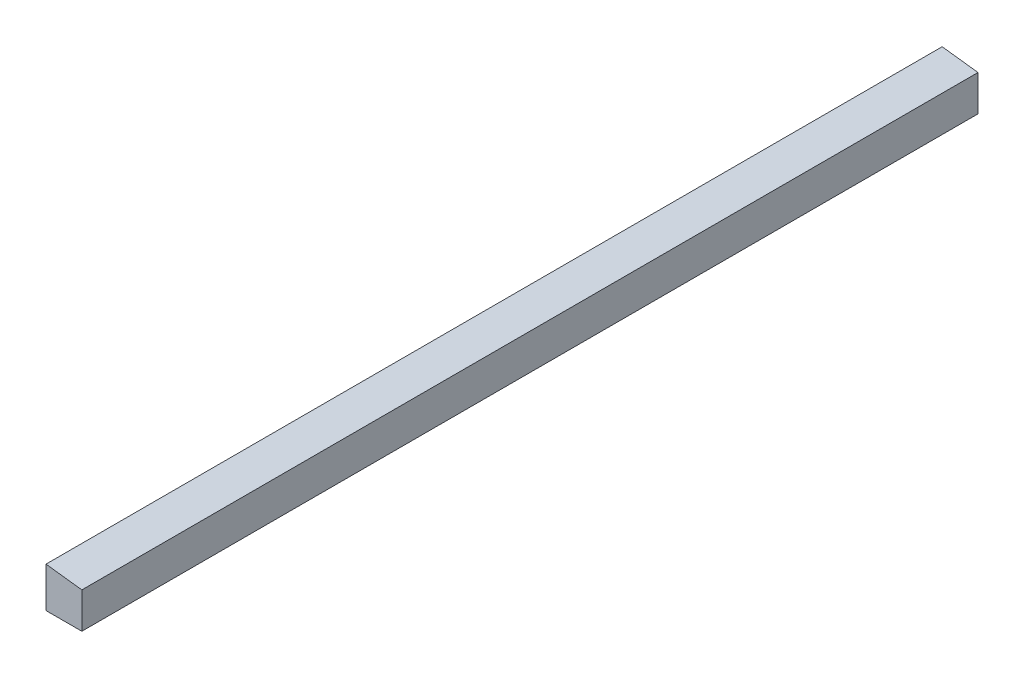
SolidWorks part; units mm, degrees
material "Plain Carbon Steel"
ref_plane "Front Plane" through (0, 0, 0) normal (0, 0, 1) x (1, 0, 0)
ref_plane "Top Plane" through (0, 0, 0) normal (0, 1, 0) x (1, 0, 0)
ref_plane "Right Plane" through (0, 0, 0) normal (1, 0, 0) x (0, 0, -1)
sketch "Sketch1" plane through (0, 0, 0) normal (0, 0, 1) x (1, 0, 0)
  line L0 (0, 0) -> (0, 11.2278)
  line L1 (0, 0) -> (10, 0)
  line L2 (10, 0) -> (10, 10)
  line L3 (10, 10) -> (0, 11.2278)
  dimension "D1" = 10
  dimension "D2" = 10
  dimension "D3" = 83
extrude "Boss-Extrude1" add sketch "Sketch1" along normal blind 250
